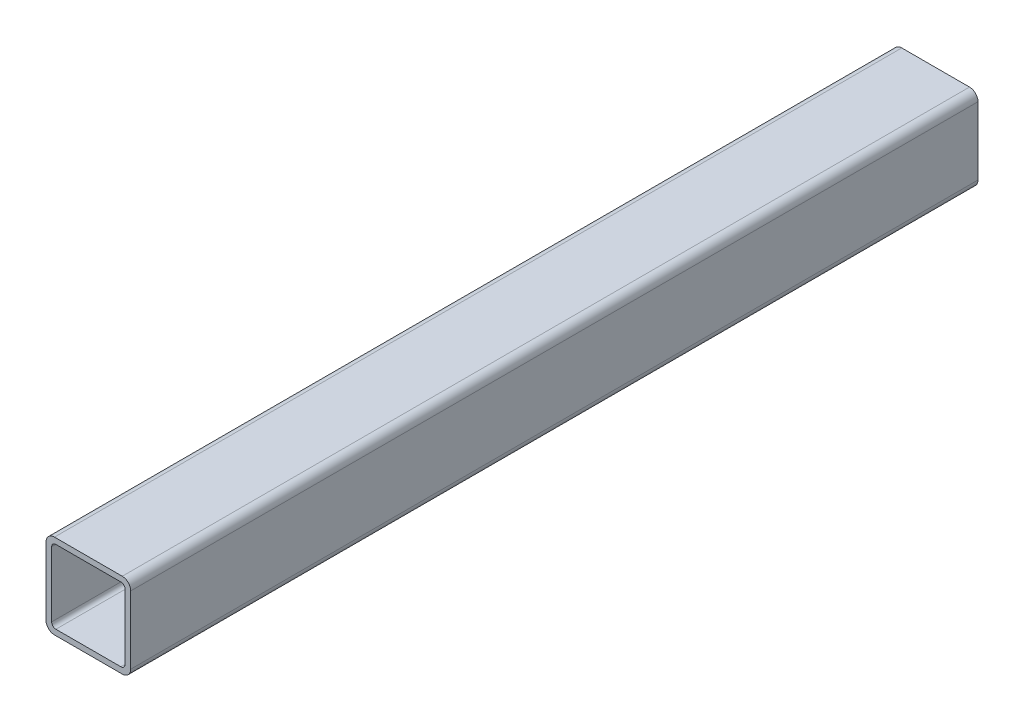
from build123d import *

# Parameters (mm, degrees)
SKETCH1_W           = 60
SKETCH1_H           = 60
SKETCH1_W_2         = 52
SKETCH1_H_2         = 52
BOSS_EXTRUDE1_DEPTH = 600
FILLET1_R           = 6
FILLET2_R           = 3


with BuildPart() as part:
    # Sketch1 → Boss-Extrude1 (new body)
    with BuildSketch(Plane.XY):
        Rectangle(SKETCH1_W, SKETCH1_H)
        Rectangle(SKETCH1_W_2, SKETCH1_H_2, mode=Mode.SUBTRACT)
    extrude(amount=BOSS_EXTRUDE1_DEPTH)

    # Fillet1
    fillet1_edges = [part.edges().sort_by_distance(p)[0] for p in [
        (30, -30, 300),
        (-30, -30, 300),
        (-30, 30, 300),
        (30, 30, 300),
    ]]
    fillet(fillet1_edges, radius=FILLET1_R)

    # Fillet2
    fillet2_edges = [part.edges().sort_by_distance(p)[0] for p in [
        (26, -26, 300),
        (26, 26, 300),
        (-26, 26, 300),
        (-26, -26, 300),
    ]]
    fillet(fillet2_edges, radius=FILLET2_R)


solid = part.part
